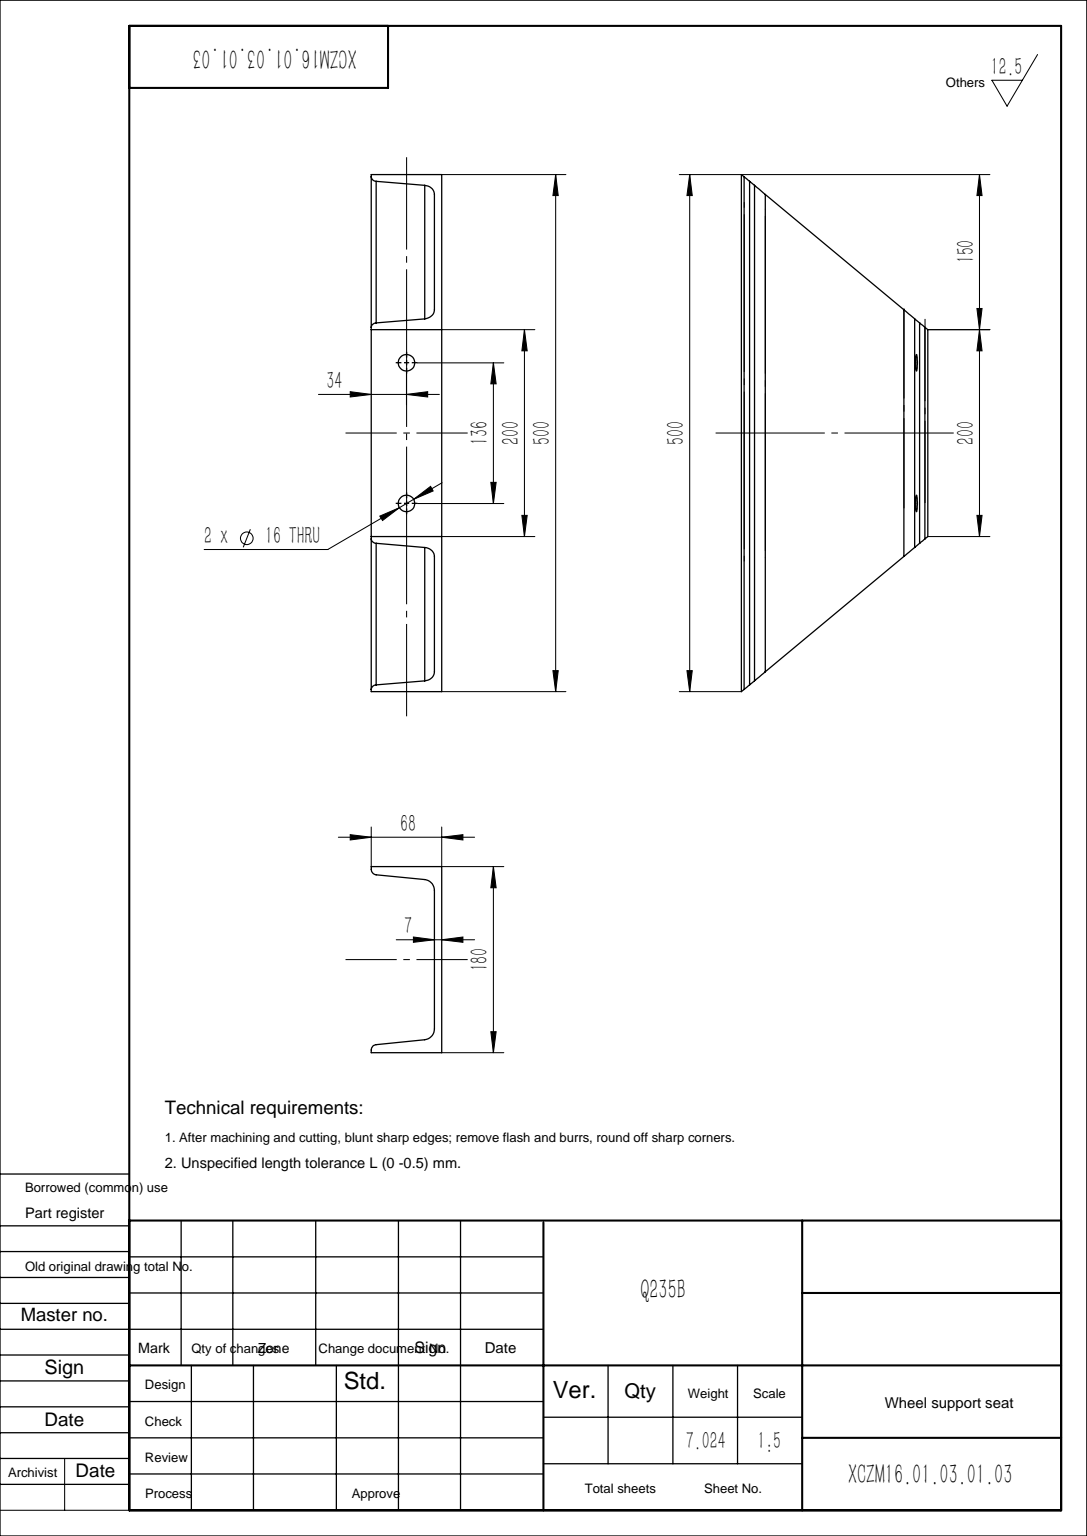
from build123d import *

# Parameters (mm, degrees)
GB_T707_1988_18A_XXXXXXXXXXXXXXX528V9_2_DEPTH = 500
CUT_EXTRUDE_1_DEPTH                           = 536.746208573
HOLE_WIZARD_16_0_16_1_REACH                   = 537.746
HOLE_WIZARD_16_0_16_1_BORE_R                  = 8


with BuildPart() as part:
    # Sketch11 → 热轧普通槽钢(gb t707-1988) 18A-XXXXXXXXXXXXXXX528V9(2) (new body)
    with BuildSketch(Plane(origin=(0, 0, 0), x_dir=(-1, 0, 0), z_dir=(0, 1, 0))):
        with BuildLine():
            Line((68, 180), (0, 180))
            Line((0, 180), (0, 0))
            Line((0, 0), (68, 0))
            Line((68, 0), (68, 2.698815299))
            ThreePointArc((68, 2.698815299), (66.642625801, 6.221593233), (63.272394525, 7.922760548))
            Line((63.272394525, 7.922760548), (16.45521095, 12.604478905))
            ThreePointArc((16.45521095, 12.604478905), (9.714748398, 16.006813534), (7, 23.052369402))
            Line((7, 23.052369402), (7, 156.947630598))
            ThreePointArc((7, 156.947630598), (9.714748398, 163.993186466), (16.45521095, 167.395521095))
            Line((16.45521095, 167.395521095), (63.272394525, 172.077239452))
            ThreePointArc((63.272394525, 172.077239452), (66.642625801, 173.778406767), (68, 177.301184701))
            Line((68, 177.301184701), (68, 180))
        make_face()
    extrude(amount=GB_T707_1988_18A_XXXXXXXXXXXXXXX528V9_2_DEPTH)

    # 草图8 → 切除-拉伸1 (cut, through all)
    with BuildSketch(Plane(origin=(0, 0, 180), x_dir=(0, 0, 1), z_dir=(-1, 0, 0))):
        Polygon((0, 500), (-180, 350), (-180, 500), align=None)
        Polygon((-180, 0), (0, 0), (-180, 150), align=None)
    extrude(amount=CUT_EXTRUDE_1_DEPTH, mode=Mode.SUBTRACT)

    # Ø16.0 (16) 直径孔1 bore → Ø16.0 (16) 直径孔1 (cut, up to next)
    with BuildSketch(Plane(origin=(0, 0, 0), x_dir=(-1, 0, 0), z_dir=(0, 0, -1)), mode=Mode.PRIVATE) as hole_wizard_16_0_16_1_sk1:
        with Locations((34, 318)):
            Circle(HOLE_WIZARD_16_0_16_1_BORE_R)
    hole_wizard_16_0_16_1_tool1 = extrude(hole_wizard_16_0_16_1_sk1.sketch, amount=-HOLE_WIZARD_16_0_16_1_REACH, mode=Mode.PRIVATE) & part.part
    # Ø16.0 (16) 直径孔1 bore → Ø16.0 (16) 直径孔1 (cut, up to next)
    with BuildSketch(Plane(origin=(0, 0, 0), x_dir=(-1, 0, 0), z_dir=(0, 0, -1)), mode=Mode.PRIVATE) as hole_wizard_16_0_16_1_sk2:
        with Locations((34, 182)):
            Circle(HOLE_WIZARD_16_0_16_1_BORE_R)
    hole_wizard_16_0_16_1_tool2 = extrude(hole_wizard_16_0_16_1_sk2.sketch, amount=-HOLE_WIZARD_16_0_16_1_REACH, mode=Mode.PRIVATE) & part.part
    add(hole_wizard_16_0_16_1_tool1.solids().sort_by_distance((-34, 318, 0))[0], mode=Mode.SUBTRACT)
    add(hole_wizard_16_0_16_1_tool2.solids().sort_by_distance((-34, 182, 0))[0], mode=Mode.SUBTRACT)


solid = part.part
